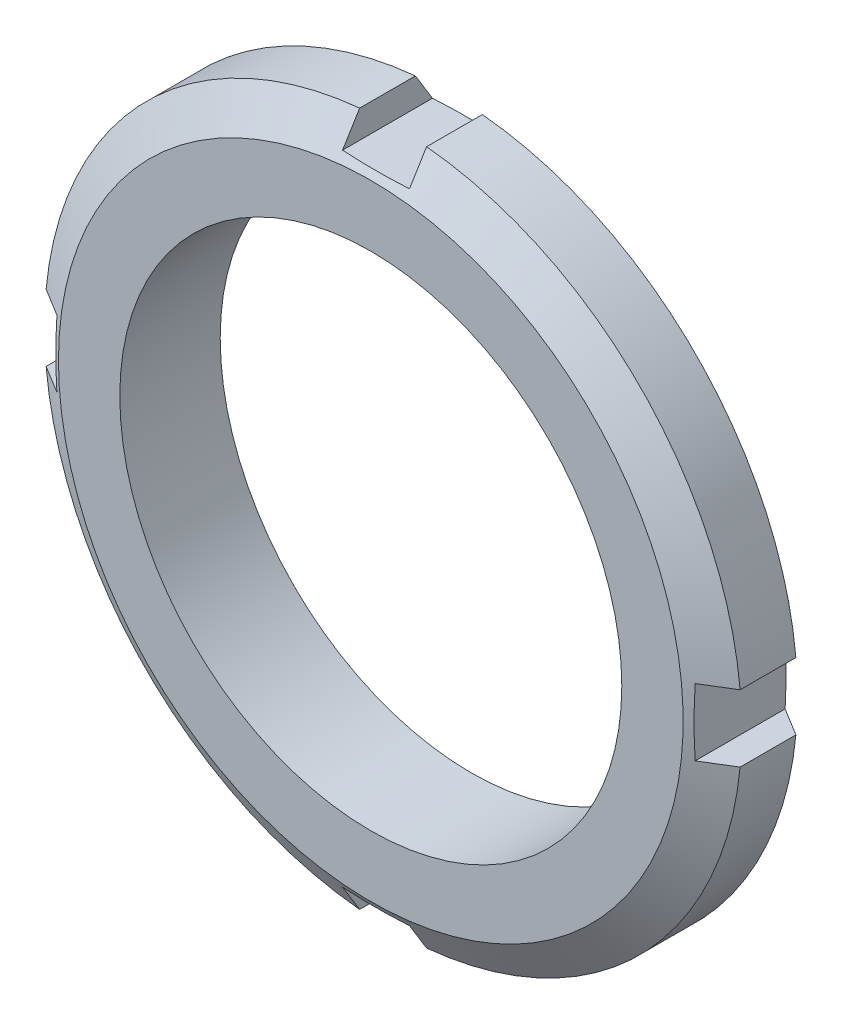
SolidWorks part; units mm, degrees
ref_plane "前视基准面" through (0, 0, 0) normal (0, 0, 1) x (1, 0, 0)
ref_plane "上视基准面" through (0, 0, 0) normal (0, 1, 0) x (1, 0, 0)
ref_plane "右视基准面" through (0, 0, 0) normal (1, 0, 0) x (0, 0, -1)
sketch "草图1" plane through (0, 0, 0) normal (0, 0, 1) x (1, 0, 0)
  circle A0 centre (0, 0) radius 62.5
  circle A1 centre (0, 0) radius 45
  dimension "D1" = 90
  dimension "D2" = 125
extrude "凸台-拉伸1" add sketch "草图1" along normal blind 18
sketch "草图2" plane through (0, 0, 0) normal (0, 1, 0) x (1, 0, 0)
  line L0 (62.5, -4) -> (62.5, 0)
  line L1 (62.5, -18) -> (62.5, 0) construction
  line L2 (62.5, 0) -> (56, 0)
  line L3 (62.5, 0) -> (-62.5, 0) construction
  line L4 (56, 0) -> (62.5, -4)
  line L5 (67.2813, -9) -> (-77.209, -9) construction
  line L6 (62.5, -14) -> (62.5, -18)
  line L7 (62.5, -18) -> (56, -18)
  line L8 (56, -18) -> (62.5, -14)
  line L9 (0, 32.6698) -> (0, -58.6969) construction
  dimension "D1" = 6.5
  dimension "D2" = 4
revolve "切除-旋转1" cut sketch "草图2" angle 360 about L9
sketch "草图3" plane through (0, 0, 0) normal (0, 0, -1) x (-1, 0, 0)
  line L0 (0, 76.897) -> (0, -80.4259) construction
  line L1 (-6, 62.2113) -> (-6, 57.2113)
  line L2 (-6, 57.2113) -> (6, 57.2113)
  line L3 (6, 57.2113) -> (6, 62.2113)
  line L4 (62.2113, 6) -> (57.2113, 6)
  line L5 (57.2113, 6) -> (57.2113, -6)
  line L6 (57.2113, -6) -> (62.2113, -6)
  line L7 (6, -62.2113) -> (6, -57.2113)
  line L8 (6, -57.2113) -> (-6, -57.2113)
  line L9 (-6, -57.2113) -> (-6, -62.2113)
  line L10 (-62.2113, -6) -> (-57.2113, -6)
  line L11 (-57.2113, -6) -> (-57.2113, 6)
  line L12 (-57.2113, 6) -> (-62.2113, 6)
  circle A0 centre (0, 0) radius 62.5 construction
  arc A1 (6, 62.2113) -> (-6, 62.2113) centre (0, 0) ccw
  arc A2 (62.2113, -6) -> (62.2113, 6) centre (0, 0) ccw
  arc A3 (-6, -62.2113) -> (6, -62.2113) centre (0, 0) ccw
  arc A4 (-62.2113, 6) -> (-62.2113, -6) centre (0, 0) ccw
  point P26 (0, 0)
  dimension "D1" = 6
  dimension "D2" = 6
  dimension "D3" = 5
  dimension "D4" = 4
extrude "切除-拉伸1" cut sketch "草图3" against normal blind 18
